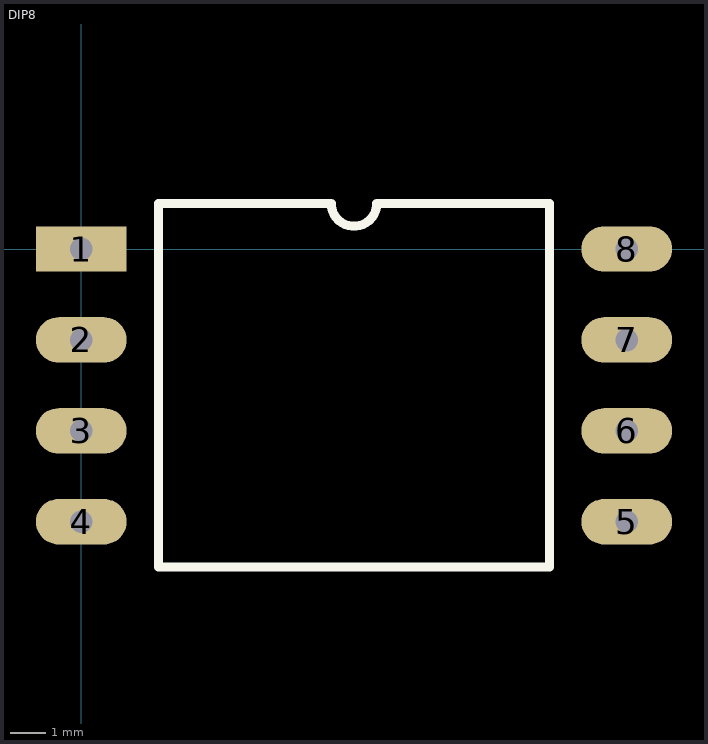
[diagram p0: the footprints below, top view; thin cyan lines are the x and y axes]
# Altium footprint library MISC89130-2.PcbLib: 2 footprints
Each footprint in its own frame and in the unit in brackets; x right, y up, seen from the top. Pads: shape width x height; smd on the part's side, far side on the other; paste and mask are expansions set on the pad; w line width, h text height; cw(c..) or ccw(c..) is an arc to the next point about the centre after c.

## DIP8 [mil]
pads (8):
  rect 100x50 hole 25: 1(0,0)
  oval 100x50 hole 25: 2(0,-100) 3(0,-200) 4(0,-300) 5(600,-300) 6(600,-200) 7(600,-100) 8(600,0)
Top Overlay:
  lines w10: 85,-350 85,50 275,50 ccw(c300,50) 325,50 515,50 515,-350 85,-350

## PCBComponent_1 [mil]